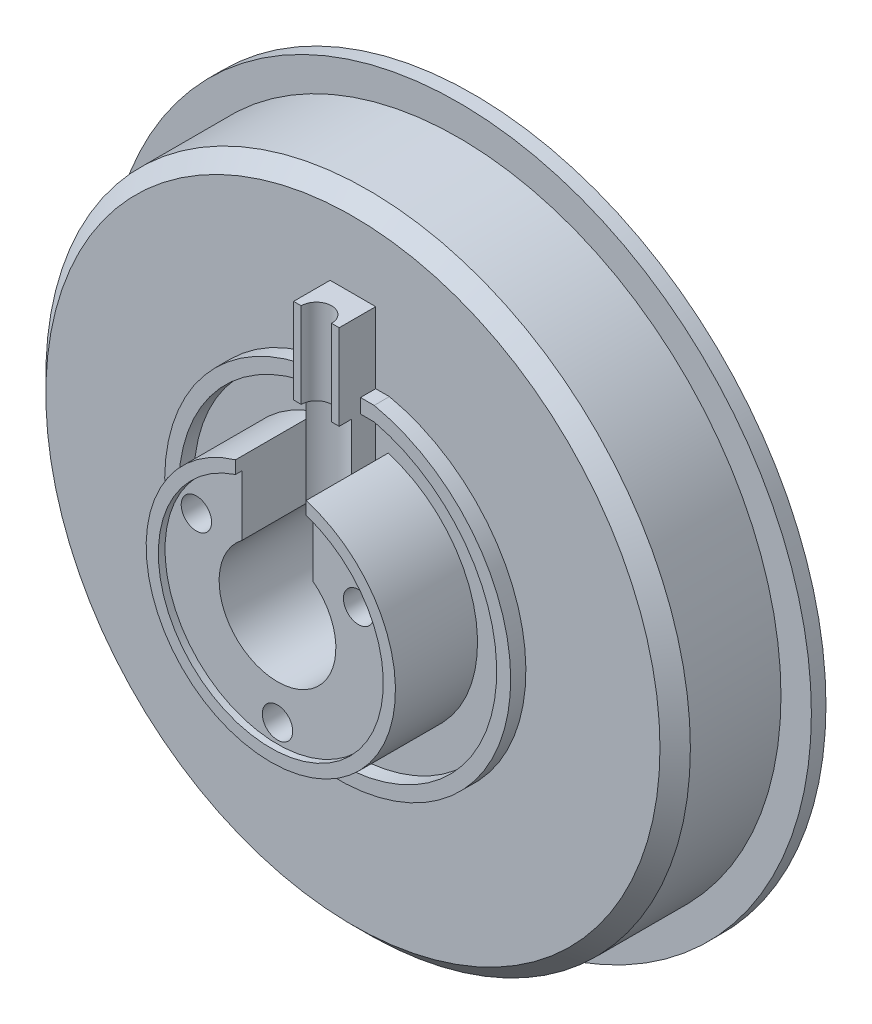
from build123d import *

# Parameters (mm, degrees)
SKETCH_1_R          = 58
EXTRUDE_1_DEPTH     = 2.4
SKETCH_2_R          = 53
EXTRUDE_2_DEPTH     = 17.4
CHAMFER_1_SIZE      = 2.5
SKETCH_3_R          = 20.5
EXTRUDE_3_DEPTH     = 13.5
SKETCH_4_R          = 18.5
CUT_EXTRUDE_1_DEPTH = 1.1
SKETCH_5_R          = 2.5
CUT_EXTRUDE_2_DEPTH = 320
SKETCH_6_R          = 50.5
CUT_EXTRUDE_3_DEPTH = 16.5
CUT_EXTRUDE_START   = -13
CUT_EXTRUDE_5_DEPTH = 13
EXTRUDE_4_DEPTH     = 2.5
SKETCH_9_W          = 11.6
SKETCH_9_H          = 21.886068862
CUT_EXTRUDE_6_DEPTH = 13.5
EXTRUDE_5_DEPTH     = 39.5
EXTRUDE_START       = -14.047642545
EXTRUDE_6_DEPTH     = 14.047642545
CUT_EXTRUDE_7_REACH = 90.118
SKETCH_10_R         = 9.6


with BuildPart() as part:
    # 草图1 → 凸台-拉伸1 (new body)
    with BuildSketch(Plane.XY):
        Circle(SKETCH_1_R)
    extrude(amount=EXTRUDE_1_DEPTH)

    # 草图2 → 凸台-拉伸2 (add)
    with BuildSketch(Plane.XY.offset(2.4)):
        Circle(SKETCH_2_R)
    extrude(amount=EXTRUDE_2_DEPTH)

    # 倒角1
    chamfer_1_edges = [part.edges().sort_by_distance(p)[0] for p in [
        (-53, 0, 19.8),
    ]]
    chamfer(chamfer_1_edges, length=CHAMFER_1_SIZE)

    # 草图3 → 凸台-拉伸3 (add)
    with BuildSketch(Plane.XY.offset(19.8)):
        Circle(SKETCH_3_R)
    extrude(amount=EXTRUDE_3_DEPTH)

    # 草图4 → 切除-拉伸1 (cut)
    with BuildSketch(Plane.XY.offset(33.3)):
        Circle(SKETCH_4_R)
    extrude(amount=-CUT_EXTRUDE_1_DEPTH, mode=Mode.SUBTRACT)

    # 草图5 → 切除-拉伸2 (cut)
    with BuildSketch(Plane.XY.offset(32.2)):
        with Locations((0, -15.4)):
            Circle(SKETCH_5_R)
        with Locations((-13.336791218, 7.7)):
            Circle(SKETCH_5_R)
        with Locations((13.336791218, 7.7)):
            Circle(SKETCH_5_R)
    extrude(amount=-CUT_EXTRUDE_2_DEPTH, mode=Mode.SUBTRACT)

    # 草图6 → 切除-拉伸3 (cut)
    with BuildSketch(Plane(origin=(0, 0, 0), x_dir=(-1, 0, 0), z_dir=(0, 0, -1))):
        Circle(SKETCH_6_R)
    extrude(amount=-CUT_EXTRUDE_3_DEPTH, mode=Mode.SUBTRACT)

    # 草图7 → 切除-拉伸5 (cut)
    with BuildSketch(Plane(origin=(0, 0, 16.5), x_dir=(-1, 0, 0), z_dir=(0, 0, -1)).offset(CUT_EXTRUDE_START)):
        with BuildLine():
            Line((-11.708521868, 0.986415561), (-17.925222851, 4.575629546))
            ThreePointArc((-17.925222851, 4.575629546), (-16.02146997, -9.25), (-5, -17.811513131))
            Line((-5, -17.811513131), (-5, -10.633085159))
            ThreePointArc((-5, -10.633085159), (-10.175798494, -5.875), (-11.708521868, 0.986415561))
        make_face()
        with BuildLine():
            Line((5, -10.633085159), (5, -17.811513131))
            ThreePointArc((5, -17.811513131), (16.02146997, -9.25), (17.925222851, 4.575629546))
            Line((17.925222851, 4.575629546), (11.708521868, 0.986415561))
            ThreePointArc((11.708521868, 0.986415561), (10.175798494, -5.875), (5, -10.633085159))
        make_face()
        with BuildLine():
            Line((-7, 9.814954576), (-12.925222851, 13.235883584))
            ThreePointArc((-12.925222851, 13.235883584), (-10.150568751, 15.466607709), (-7, 17.12454379))
            Line((-7, 17.12454379), (-7, 9.814954576))
        make_face()
        with BuildLine():
            Line((7, 9.814954576), (12.925222851, 13.235883584))
            ThreePointArc((12.925222851, 13.235883584), (10.150568751, 15.466607709), (7, 17.12454379))
            Line((7, 17.12454379), (7, 9.814954576))
        make_face()
    extrude(amount=CUT_EXTRUDE_5_DEPTH, mode=Mode.SUBTRACT)

    # 草图8 → 凸台-拉伸4 (add)
    with BuildSketch(Plane.XY.offset(19.8)):
        with BuildLine():
            Line((-6, 27.810115066), (6, 27.810115066))
            ThreePointArc((6, 27.810115066), (0, -28.45), (-6, 27.810115066))
        make_face()
        with BuildLine():
            Line((-6, 25.452357455), (6, 25.452357455))
            ThreePointArc((6, 25.452357455), (0, -26.15), (-6, 25.452357455))
        make_face(mode=Mode.SUBTRACT)
    extrude(amount=EXTRUDE_4_DEPTH)

    # 草图9 → 切除-拉伸6 (cut)
    with BuildSketch(Plane.XY.offset(33.3)):
        with Locations((0, 10.943034431)):
            Rectangle(SKETCH_9_W, SKETCH_9_H)
    extrude(amount=-CUT_EXTRUDE_6_DEPTH, mode=Mode.SUBTRACT)

    # 草图11 → 凸台-拉伸5 (add)
    with BuildSketch(Plane(origin=(0, 0, 0), x_dir=(1, 0, 0), z_dir=(0, 1, 0))):
        with BuildLine():
            Line((-3.75, -19.8), (3.75, -19.8))
            Line((3.75, -19.8), (3.75, -23.8))
            ThreePointArc((3.75, -23.8), (0, -21.8), (-3.75, -23.8))
            Line((-3.75, -23.8), (-3.75, -19.8))
        make_face()
    extrude(amount=EXTRUDE_5_DEPTH)

    # 草图12 → 凸台-拉伸6 (add)
    with BuildSketch(Plane(origin=(0, 39.5, 0), x_dir=(1, 0, 0), z_dir=(0, 1, 0)).offset(EXTRUDE_START)):
        with BuildLine():
            Line((-3.75, -23.8), (-3.75, -25.8))
            Line((-3.75, -25.8), (-2.5, -25.8))
            ThreePointArc((-2.5, -25.8), (0, -23.3), (2.5, -25.8))
            Line((2.5, -25.8), (3.75, -25.8))
            Line((3.75, -25.8), (3.75, -23.8))
            ThreePointArc((3.75, -23.8), (0, -21.8), (-3.75, -23.8))
        make_face()
    extrude(amount=EXTRUDE_6_DEPTH)

    # 草图10 → 切除-拉伸7 (cut, up to next)
    with BuildSketch(Plane.XY.offset(32.2), mode=Mode.PRIVATE) as cut_extrude_7_sk1:
        with Locations(Location((0, 0, 0), (0, 0, 52.831100344))):
            Circle(SKETCH_10_R)
    cut_extrude_7_tool1 = extrude(cut_extrude_7_sk1.sketch, amount=-CUT_EXTRUDE_7_REACH, mode=Mode.PRIVATE) & part.part
    add(cut_extrude_7_tool1.solids().sort_by_distance((0, 0, 32.2))[0], mode=Mode.SUBTRACT)


solid = part.part
